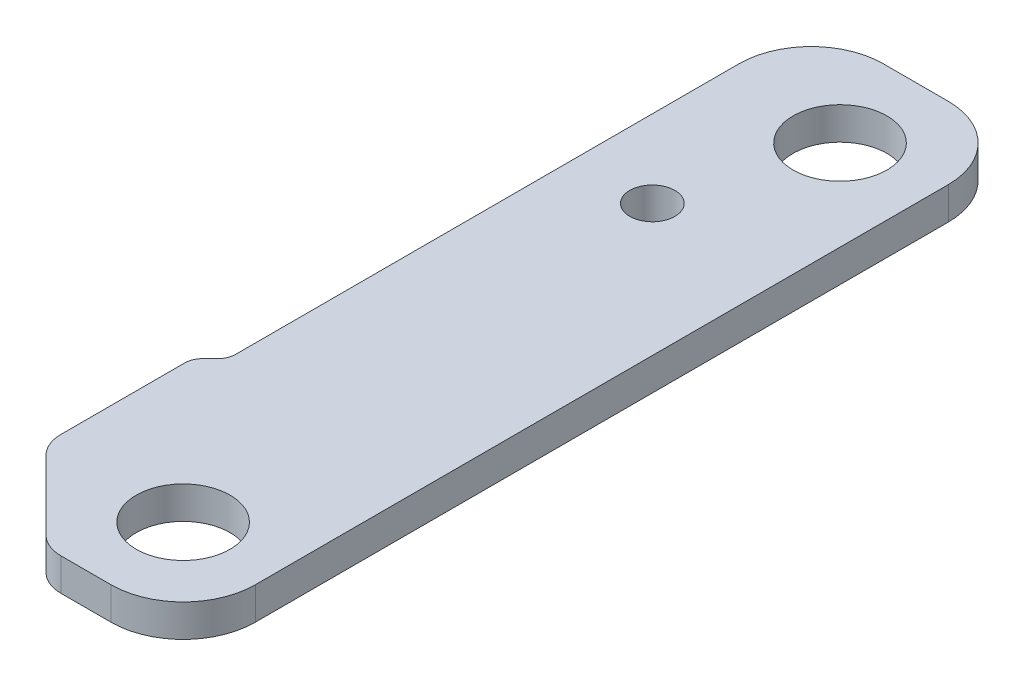
SolidWorks part; units mm, degrees
ref_plane "Front Plane" through (0, 0, 0) normal (0, 0, 1) x (1, 0, 0)
ref_plane "Top Plane" through (0, 0, 0) normal (0, 1, 0) x (1, 0, 0)
ref_plane "Right Plane" through (0, 0, 0) normal (1, 0, 0) x (0, 0, -1)
sketch "Sketch1" plane through (0, 0, 0) normal (0, 1, 0) x (1, 0, 0)
  line L0 (2.9289, 22.0711) -> (22.0711, 2.9289)
  line L1 (29.1421, 0) -> (43, 0)
  line L2 (63, 20) -> (63, 212)
  line L3 (0, 29.1421) -> (0, 63.4289)
  line L4 (1.4645, 66.9645) -> (3.5355, 69.0355)
  line L5 (5, 72.5711) -> (5, 212)
  line L6 (25, 232) -> (43, 232)
  arc A0 (3.5355, 69.0355) -> (5, 72.5711) centre (0, 72.5711) ccw
  arc A1 (0, 63.4289) -> (1.4645, 66.9645) centre (5, 63.4289) cw
  arc A2 (63, 20) -> (43, 0) centre (43, 20) cw
  circle A3 centre (38, 25) radius 13
  circle A4 centre (38, 207) radius 13
  arc A5 (5, 212) -> (25, 232) centre (25, 212) cw
  arc A6 (63, 212) -> (43, 232) centre (43, 212) ccw
  arc A7 (2.9289, 22.0711) -> (0, 29.1421) centre (10, 29.1421) cw
  arc A8 (22.0711, 2.9289) -> (29.1421, 0) centre (29.1421, 10) ccw
  circle A9 centre (26.5, 166.5) radius 6.25
  point P0 (0, 0)
  point P9 (5, 70.5)
  point P12 (63, 0)
  point P19 (0, 65.5)
  point P22 (63, 0)
  point P27 (63, 232)
  point P30 (0, 25)
  point P33 (25, 0)
  dimension "D3" = 5
  dimension "D4" = 5
  dimension "D5" = 232
  dimension "D7" = 26
  dimension "D8" = 26
  dimension "D9" = 38
  dimension "D10" = 0
  dimension "D1" = 65.5
  dimension "D11" = 182
  dimension "D12" = 25
  dimension "D13" = 5
  dimension "D14" = 20
  dimension "D15" = 10
  dimension "D16" = 11.5
  dimension "D17" = 141.5
  dimension "D2" = 63
extrude "Boss-Extrude1" add sketch "Sketch1" along normal blind 9
